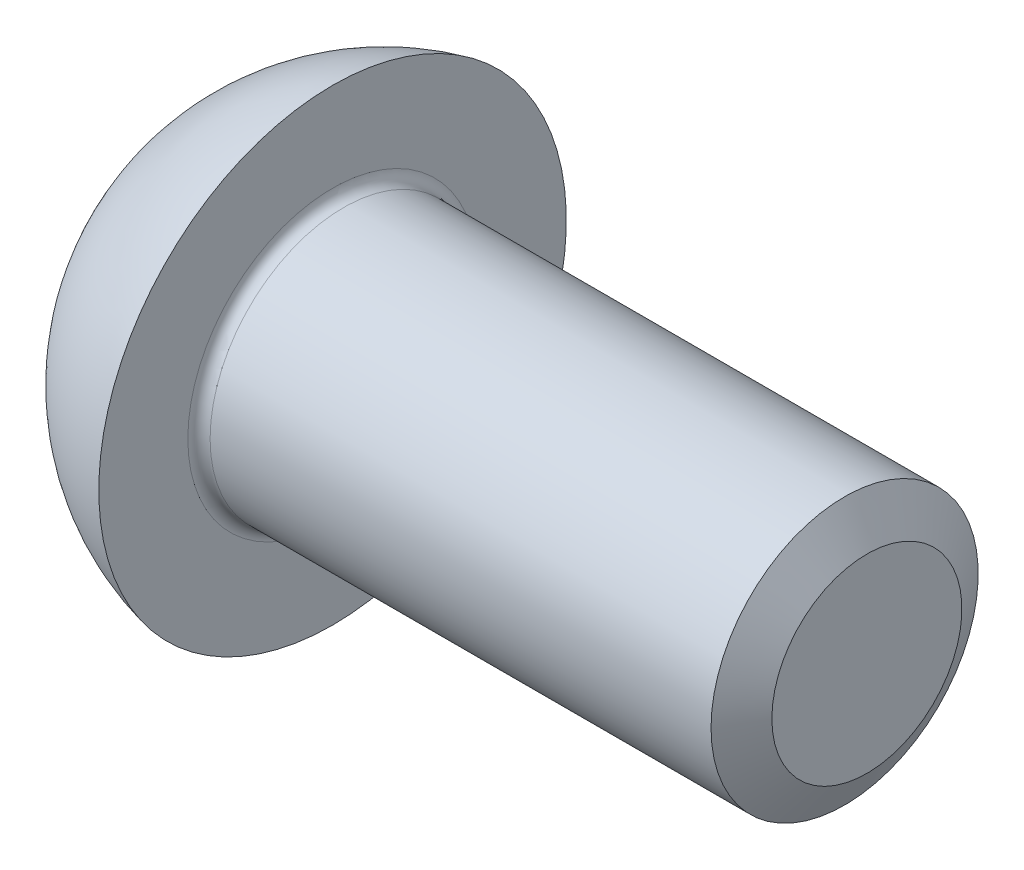
from build123d import *

# Parameters (mm, degrees)
CUT_EXTRUDE1_DEPTH = 3.3


with BuildPart() as part:
    # Sketch1 → Revolve1 (revolve)
    with BuildSketch(Plane.XY, mode=Mode.PRIVATE) as revolve1_sk:
        with BuildLine():
            Line((0, 3), (-11.75, 3))
            ThreePointArc((-11.75, 3), (-11.926776695, 3.073223305), (-12, 3.25))
            Line((-12, 3.25), (-12, 5.25))
            ThreePointArc((-12, 5.25), (-13.866655204, 4.442760966), (-15.3, 3))
            Line((-15.3, 3), (-15.3, 0))
            Line((-15.3, 0), (0, 0))
            Line((0, 0), (0, 3))
        make_face()
    revolve(revolve1_sk.sketch.rotate(Axis((-15.3, 0, 0), (1, 0, 0)), 90), axis=Axis((-15.3, 0, 0), (1, 0, 0)))

    # Sketch2 → Cut-Extrude1 (cut)
    with BuildSketch(Plane.ZY.offset(15.3)):
        Polygon((0, 2.309401077), (-2, 1.154700538), (-2, -1.154700538), (0, -2.309401077), (2, -1.154700538), (2, 1.154700538), align=None)
    extrude(amount=-CUT_EXTRUDE1_DEPTH, mode=Mode.SUBTRACT)

    # Sketch6 → Revolve2 (revolve)
    with BuildSketch(Plane.XY):
        Polygon((-13.22, 2.309401077), (-12, 0), (-11.42, 0), (-11.42, 2.309401077), align=None)
    revolve(axis=Axis((-15.3, 0, 0), (1, 0, 0)))

    # Sketch7 → Cut-Revolve5 (revolve, cut)
    with BuildSketch(Plane.XY):
        Polygon((-15.3, 2.309401077), (-14.72, 0), (-15.3, 0), align=None)
    revolve(axis=Axis((-15.3, 0, 0), (1, 0, 0)), mode=Mode.SUBTRACT)

    # Sketch4 → Cut-Revolve1 (revolve, cut)
    with BuildSketch(Plane.XY, mode=Mode.PRIVATE) as cut_revolve1_sk:
        Polygon((-0.5, 3), (0, 2.133974596), (0.5, 3), align=None)
    revolve(cut_revolve1_sk.sketch.rotate(Axis((-0.5, 0, 0), (1, 0, 0)), 90), axis=Axis((-0.5, 0, 0), (1, 0, 0)), mode=Mode.SUBTRACT)


solid = part.part
